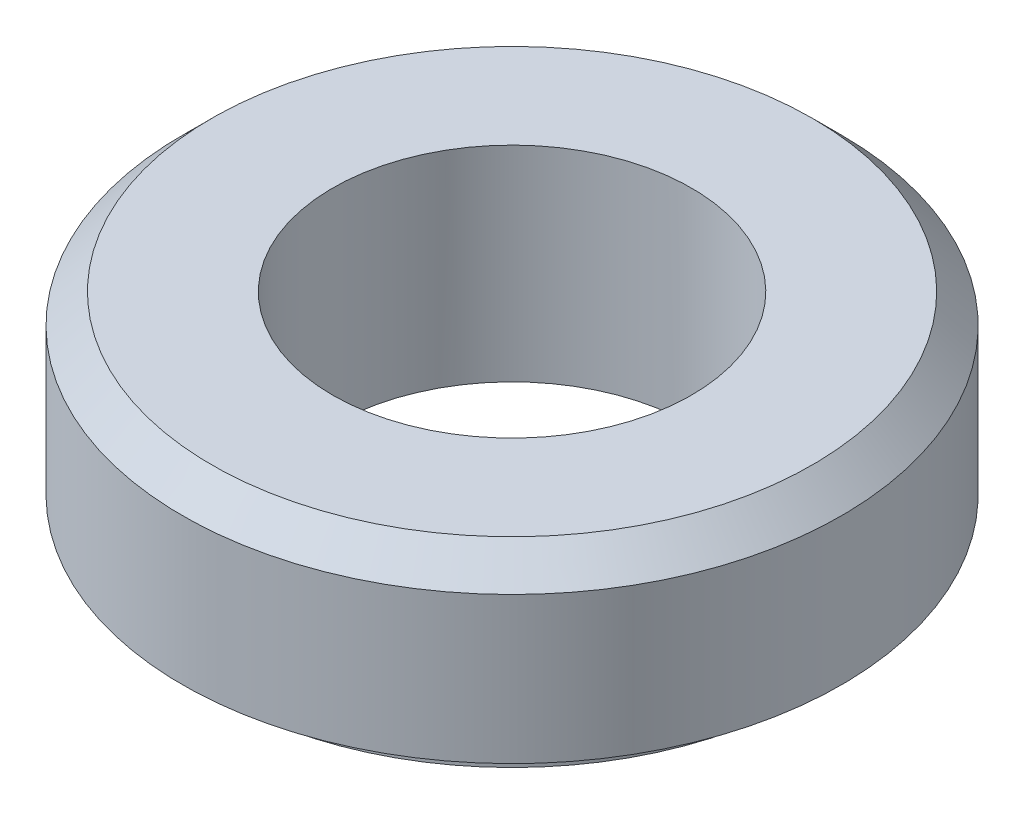
SolidWorks part; units mm, degrees
material "Q235B"
ref_plane "Front Plane" through (0, 0, 0) normal (0, 0, 1) x (1, 0, 0)
ref_plane "Top Plane" through (0, 0, 0) normal (0, 1, 0) x (1, 0, 0)
ref_plane "Right Plane" through (0, 0, 0) normal (1, 0, 0) x (0, 0, -1)
sketch "Sketch1" plane through (0, 0, 0) normal (1, 0, 0) x (0, 0, -1)
  line L0 (0, 0) -> (0, 14) construction
  line L1 (20, 0) -> (20, 2)
  line L2 (20, 2) -> (22.5, 2)
  line L3 (22.5, 2) -> (22.5, 12)
  line L4 (20.5, 14) -> (12, 14)
  line L5 (12, 14) -> (12, 0)
  line L6 (12, 0) -> (20, 0)
  line L7 (22.5, 12) -> (20.5, 14)
  point P5 (22.5, 14)
  dimension "D1" = 24
  dimension "D2" = 40
  dimension "D3" = 45
  dimension "D4" = 2
  dimension "D5" = 12
revolve "Revolve1" add sketch "Sketch1" angle 360 about L0
hole_wizard "G3/4 Tapped Hole1" positions "Sketch4" profile "Sketch5" tap size "G3/4" standard "GB"
sketch "Sketch4" plane through (0, 14, 0) normal (0, 1, 0) x (1, 0, 0)
  point P0 (0, 0)
sketch "Sketch5" plane through (0, 14, 0) normal (1, 0, 0) x (0, 0, 1)
  line L0 (0, 0) -> (0, 65.6805)
  line L1 (0, 65.6805) -> (12.25, 58.32)
  line L2 (12.25, 58.32) -> (12.25, 0)
  line L5 (12.25, 0) -> (0, 0)
  line L10 (0, 65.6805) -> (-12.25, 58.32) construction
  line L11 (0, -6.35) -> (0, 107.95) construction
  dimension "螺纹孔钻头直径" = 24.5
  dimension "螺纹孔钻头深度" = 58.32
  dimension "导头角度" = 118
cosmetic thread "Hole Cosmetic Thread2"
